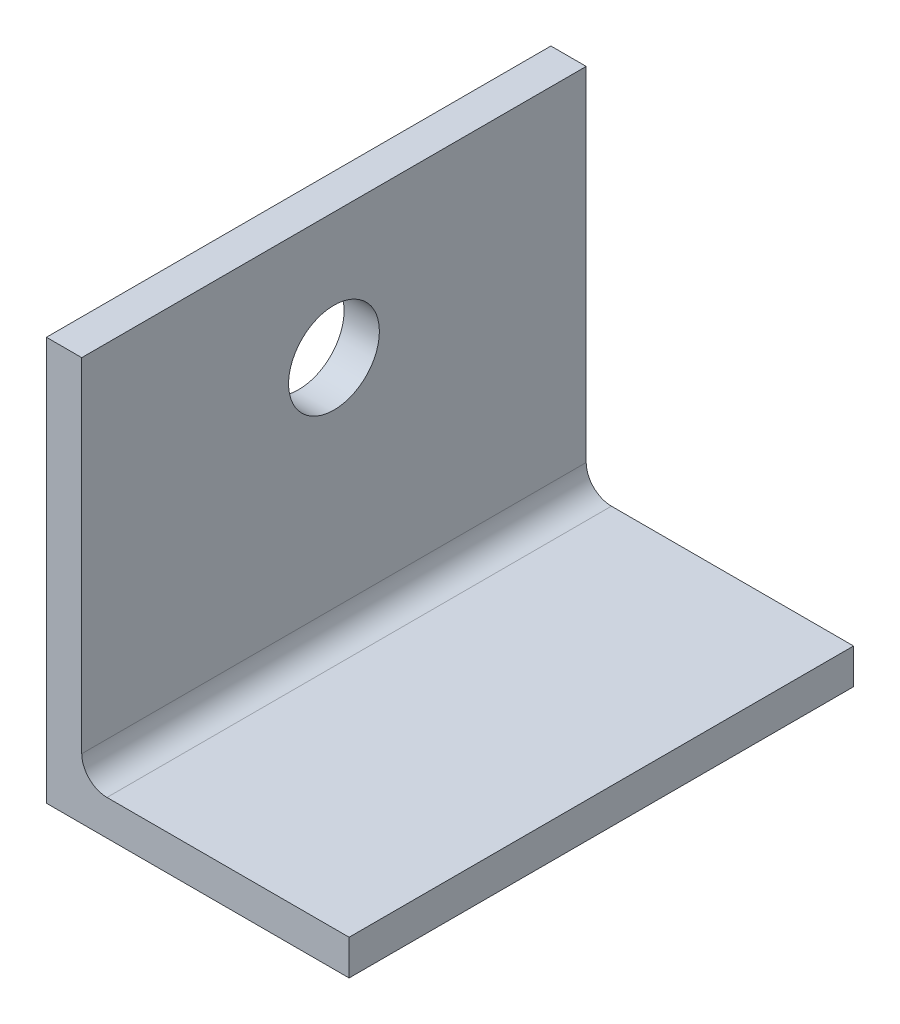
SolidWorks part; units mm, degrees
material "1023 碳钢板 (SS)"
ref_plane "Front Plane" through (0, 0, 0) normal (0, 0, 1) x (1, 0, 0)
ref_plane "Top Plane" through (0, 0, 0) normal (0, 1, 0) x (1, 0, 0)
ref_plane "Right Plane" through (0, 0, 0) normal (1, 0, 0) x (0, 0, -1)
sketch "Sketch1" plane through (0, 0, 0) normal (0, 0, 1) x (1, 0, 0)
  line L0 (0, 0) -> (0, -80)
  line L1 (0, -80) -> (60, -80)
  line L2 (7, 0) -> (7, -73)
  line L3 (7, -73) -> (60, -73)
  line L4 (7, 0) -> (0, 0)
  line L5 (60, -73) -> (60, -80)
  dimension "D1" = 60
  dimension "D2" = 80
  dimension "D3" = 7
extrude "Boss-Extrude1" add sketch "Sketch1" along normal blind 100
sketch "Sketch2" plane through (7, 0, 0) normal (1, 0, 0) x (0, 0, -1)
  line L0 (-100, -73) -> (-100, 0) construction
  line L1 (-100, -80) -> (0, -80) construction
  circle A0 centre (-50, -25) radius 9
  dimension "D1" = 18
  dimension "D3" = 55
  dimension "D2" = 50
extrude "Cut-Extrude1" cut sketch "Sketch2" against normal blind 100
fillet "Fillet1" radius 5 1 edges at (7, -73, 50)
